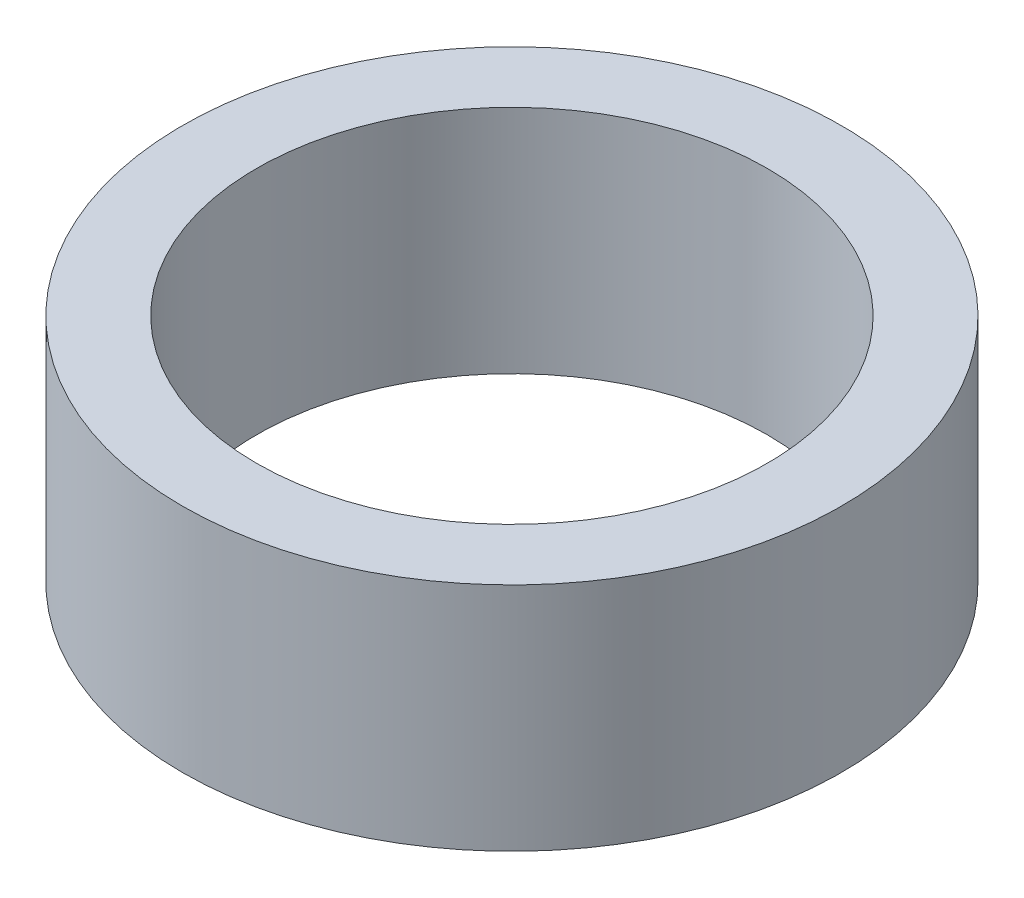
from build123d import *

# Parameters (mm, degrees)
SKETCH1_R           = 4
SKETCH1_R_2         = 3.1
BOSS_EXTRUDE1_DEPTH = 2.8


with BuildPart() as part:
    # Sketch1 → Boss-Extrude1 (new body)
    with BuildSketch(Plane(origin=(0, 0, 0), x_dir=(1, 0, 0), z_dir=(0, 1, 0))):
        with Locations(Location((0, 0, 0), (0, 0, 270))):
            Circle(SKETCH1_R)
        with Locations(Location((0, 0, 0), (0, 0, 270))):
            Circle(SKETCH1_R_2, mode=Mode.SUBTRACT)
    extrude(amount=BOSS_EXTRUDE1_DEPTH)


solid = part.part
